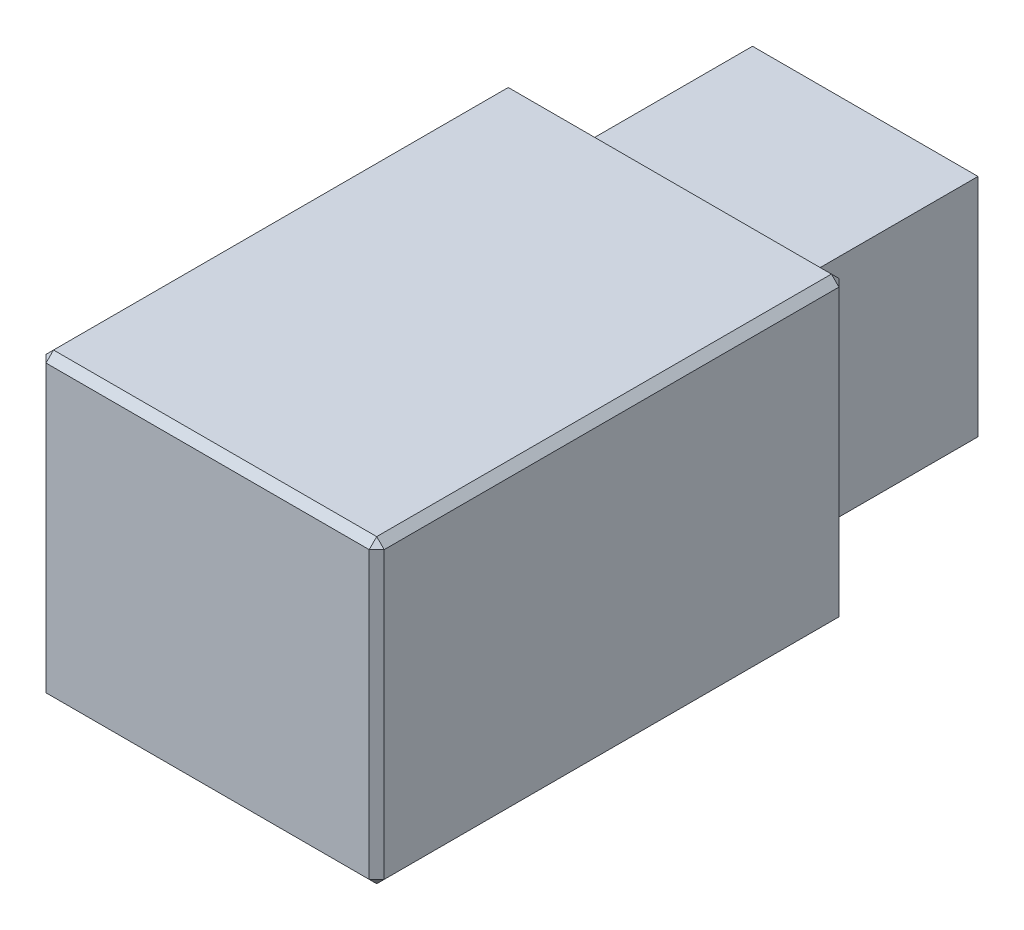
SolidWorks part; units mm, degrees
ref_plane "前视" through (0, 0, 0) normal (0, 0, 1) x (1, 0, 0)
ref_plane "上视" through (0, 0, 0) normal (0, 1, 0) x (1, 0, 0)
ref_plane "右视" through (0, 0, 0) normal (1, 0, 0) x (0, 0, -1)
sketch "草图1" plane through (0, 0, 0) normal (0, 0, 1) x (1, 0, 0)
  line L1 (0, 0) -> (60, 0)
  line L2 (0, 0) -> (0, 60)
  line L3 (0, 60) -> (60, 60)
  line L4 (60, 0) -> (60, 60)
  dimension "D1" = 60
  dimension "D2" = 60
extrude "基体-拉伸" add sketch "草图1" along normal blind 50
sketch "草图2" plane through (0, 0, 50) normal (0, 0, 1) x (1, 0, 0)
  line L0 (0, 60) -> (0, 0) construction
  line L1 (-15, 70) -> (75, 70)
  line L2 (-15, 70) -> (-15, -10)
  line L3 (-15, -10) -> (75, -10)
  line L4 (75, 70) -> (75, -10)
  line L5 (60, 0) -> (60, 60) construction
  line L6 (60, 60) -> (0, 60) construction
  line L7 (0, 0) -> (60, 0) construction
  dimension "D1" = 15
  dimension "D2" = 15
  dimension "D3" = 10
  dimension "D4" = 10
extrude "凸台-拉伸1" add sketch "草图2" along normal blind 125
chamfer "倒角1" distance 2 angle 45
sketch "草图3" plane through (0, 0, 0) normal (0, 0, -1) x (-1, 0, 0)
  line L0 (-60, 0) -> (-60, 60) construction
  line L1 (0, 0) -> (-60, 0) construction
  circle A0 centre (-30, 30) radius 6
  dimension "D1" = 12
  dimension "D2" = 30
  dimension "D3" = 30
extrude "切除-拉伸1" cut sketch "草图3" against normal blind 80
